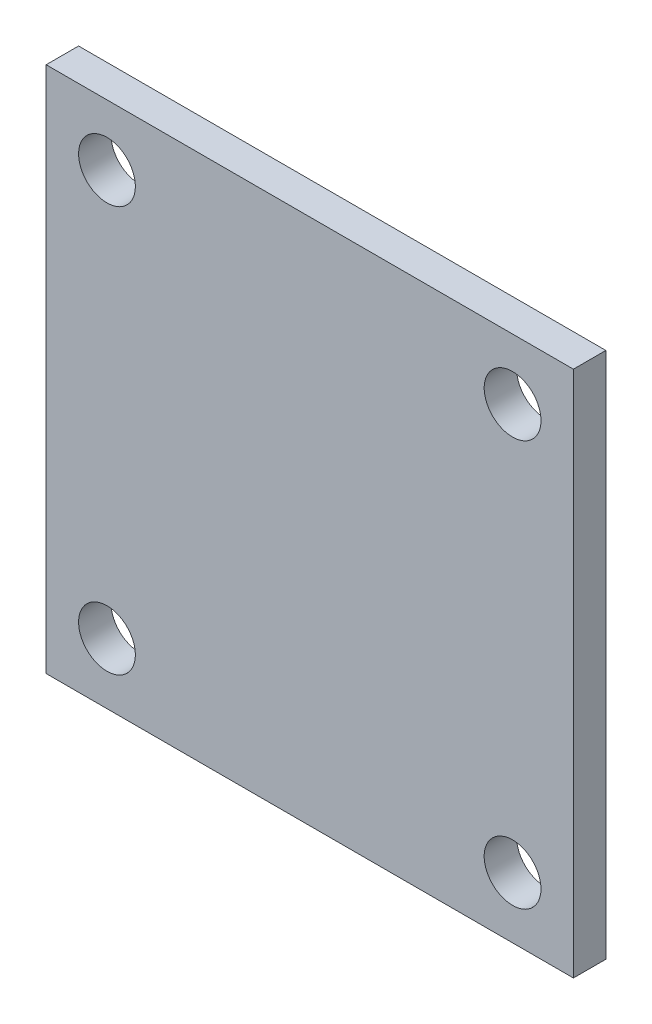
SolidWorks part; units mm, degrees
material "Q235B"
ref_plane "Front Plane" through (0, 0, 0) normal (0, 0, 1) x (1, 0, 0)
ref_plane "Top Plane" through (0, 0, 0) normal (0, 1, 0) x (1, 0, 0)
ref_plane "Right Plane" through (0, 0, 0) normal (1, 0, 0) x (0, 0, -1)
other "Configuration Table"
sketch "Sketch1" plane through (0, 0, 0) normal (0, 0, 1) x (1, 0, 0)
  line L1 (-65, -65) -> (65, -65)
  line L2 (-65, -65) -> (-65, 65)
  line L3 (-65, 65) -> (65, 65)
  line L4 (65, -65) -> (65, 65)
  line L5 (-65, -65) -> (65, 65) construction
  line L6 (-65, 65) -> (65, -65) construction
  circle A0 centre (-50, 50) radius 7
  circle A1 centre (50, 50) radius 7
  circle A2 centre (50, -50) radius 7
  circle A3 centre (-50, -50) radius 7
  point P0 (0, 0)
  point P11 (0, 0)
  point P14 (0, 0)
  point P17 (0, 0)
  point P20 (0, 0)
  dimension "D4" = 14
  dimension "D1" = 130
  dimension "D2" = 130
  dimension "D3" = 50
  dimension "D5" = 4
extrude "Boss-Extrude1" add sketch "Sketch1" along normal blind 8
